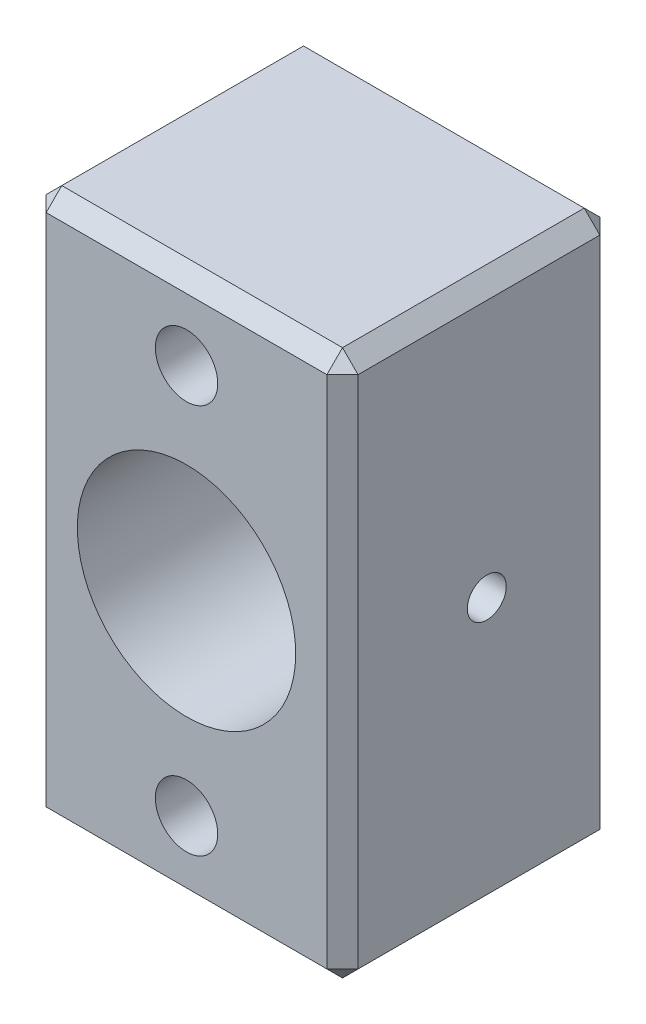
from build123d import *

# Parameters (mm, degrees)
SKETCH_1_W              = 40
SKETCH_1_H              = 70
EXTRUDE_1_DEPTH         = 35
SKETCH_2_R              = 14
CUT_EXTRUDE_1_DEPTH     = 64
SKETCH_4_R              = 4
CUT_EXTRUDE_3_DEPTH     = 59
HOLE_WIZARD_M6_1_REACH  = 58.279
HOLE_WIZARD_M6_1_BORE_R = 2.5
CHAMFER_1_SIZE          = 2


with BuildPart() as part:
    # 草图1 → 凸台-拉伸1 (new body)
    with BuildSketch(Plane.XY):
        Rectangle(SKETCH_1_W, SKETCH_1_H)
    extrude(amount=EXTRUDE_1_DEPTH)

    # 草图2 → 切除-拉伸1 (cut)
    with BuildSketch(Plane.XY.offset(35)):
        Circle(SKETCH_2_R)
    extrude(amount=-CUT_EXTRUDE_1_DEPTH, mode=Mode.SUBTRACT)

    # 草图4 → 切除-拉伸3 (cut)
    with BuildSketch(Plane.XY.offset(35)):
        with Locations((0, 25)):
            Circle(SKETCH_4_R)
    cut_extrude_3 = extrude(amount=-CUT_EXTRUDE_3_DEPTH, mode=Mode.SUBTRACT)

    # M6 螺纹孔1 bore (on position points) → M6 螺纹孔1 (cut, up to next)
    with BuildSketch(Plane(origin=(-20, 0, 16.498820141), x_dir=(0, 0, -1), z_dir=(-1, 0, 0)), mode=Mode.PRIVATE) as hole_wizard_m6_1_sk1:
        Circle(HOLE_WIZARD_M6_1_BORE_R)
    hole_wizard_m6_1_tool1 = extrude(hole_wizard_m6_1_sk1.sketch, amount=-HOLE_WIZARD_M6_1_REACH, mode=Mode.PRIVATE) & part.part
    hole_wizard_m6_1 = hole_wizard_m6_1_tool1.solids().sort_by_distance((-20, 0, 16.49882))[0]
    add(hole_wizard_m6_1, mode=Mode.SUBTRACT)

    # 镜向2: 切除-拉伸3 across plane
    add(cut_extrude_3.mirror(Plane.ZX), mode=Mode.SUBTRACT)

    # 镜向3: M6 螺纹孔1 across plane
    add(hole_wizard_m6_1.mirror(Plane(origin=(0, 0, 0), x_dir=(0, 0, 1), z_dir=(1, 0, 0))), mode=Mode.SUBTRACT)

    # 倒角1
    chamfer_1_edges = [part.edges().sort_by_distance(p)[0] for p in [
        (-20, 0, 35),
        (0, -35, 35),
        (20, 0, 35),
        (0, -35, 0),
        (-20, 0, 0),
        (0, 35, 0),
        (20, 0, 0),
        (20, -35, 17.5),
        (-20, -35, 17.5),
        (-20, 35, 17.5),
        (20, 35, 17.5),
        (0, 35, 35),
    ]]
    chamfer(chamfer_1_edges, length=CHAMFER_1_SIZE)


solid = part.part
